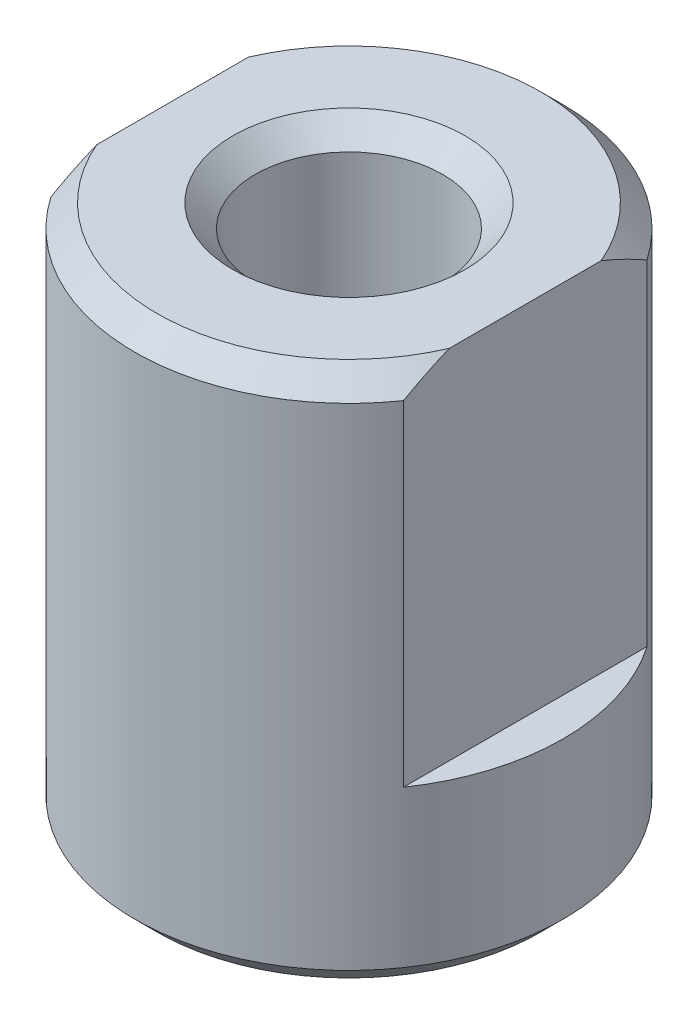
SolidWorks part; units mm, degrees
material "SUS 303"
ref_plane "Front Plane" through (0, 0, 0) normal (0, 0, 1) x (1, 0, 0)
ref_plane "Top Plane" through (0, 0, 0) normal (0, 1, 0) x (1, 0, 0)
ref_plane "Right Plane" through (0, 0, 0) normal (1, 0, 0) x (0, 0, -1)
sketch "Sketch1" plane through (0, 0, 0) normal (0, 0, 1) x (1, 0, 0)
  line L0 (0, 12) -> (0, 24.1121) construction
  line L1 (0, 0) -> (4.3, 0)
  line L2 (0, 0) -> (0, 12)
  line L3 (0, 12) -> (4.3, 12)
  line L4 (4.8, 0.5) -> (4.8, 11.5)
  line L5 (4.3, 12) -> (4.8, 11.5)
  line L6 (4.3, 0) -> (4.8, 0.5)
  point P1 (4.8, 12)
  point P3 (4.8, 0)
  dimension "D1" = 4.8
  dimension "D2" = 12
revolve "Revolve1" add sketch "Sketch1" angle 360 about L0
hole_wizard "M5 Tapped Hole1" positions "Sketch2" profile "Sketch3" tap size "M5" standard "GB" end condition through all
sketch "Sketch2" plane through (0, 12, 0) normal (0, 1, 0) x (1, 0, 0)
  point P0 (0, 0)
sketch "Sketch3" plane through (0, 12, 0) normal (1, 0, 0) x (0, 0, 1)
  line L0 (0, 0) -> (0, 12)
  line L1 (0, 12) -> (2.6, 12)
  line L2 (2.1, 11.5) -> (2.1, 0.5)
  line L3 (2.1, 0.5) -> (2.6, 0)
  line L5 (2.6, 0) -> (0, 0)
  line L6 (-2.1, 0.5) -> (-2.6, 0) construction
  line L7 (2.6, 12) -> (2.1, 11.5)
  line L8 (-2.6, 12) -> (-2.1, 11.5) construction
  line L11 (0, -6.35) -> (0, 107.95) construction
  dimension "通孔螺纹孔钻头直径" = 4.2
  dimension "通孔螺纹孔钻头深度" = 12
  dimension "近端锥形沉头孔直径" = 5.2
  dimension "近端锥形沉头孔角度" = 90
  dimension "远端锥形沉头孔直径" = 5.2
  dimension "远端锥形沉头孔角度" = 90
cosmetic thread "Cosmetic Thread2"
sketch "Sketch4" plane through (0, 0, 0) normal (0, 0, 1) x (1, 0, 0)
  line L0 (0, 0) -> (0, 6.4585) construction
  line L1 (-5.3339, 12) -> (-3.95, 12)
  line L2 (-5.3339, 12) -> (-5.3339, 4)
  line L3 (-5.3339, 4) -> (-3.95, 4)
  line L4 (-3.95, 12) -> (-3.95, 4)
  line L5 (-4.3, 0) -> (4.3, 0) construction
  line L7 (3.95, 12) -> (3.95, 4)
  line L8 (5.3339, 4) -> (3.95, 4)
  line L9 (5.3339, 12) -> (5.3339, 4)
  line L10 (5.3339, 12) -> (3.95, 12)
  dimension "D1" = 7.9
  dimension "D2" = 4
  dimension "D3" = 8
extrude "Cut-Extrude1" cut sketch "Sketch4" against normal mid plane 10
